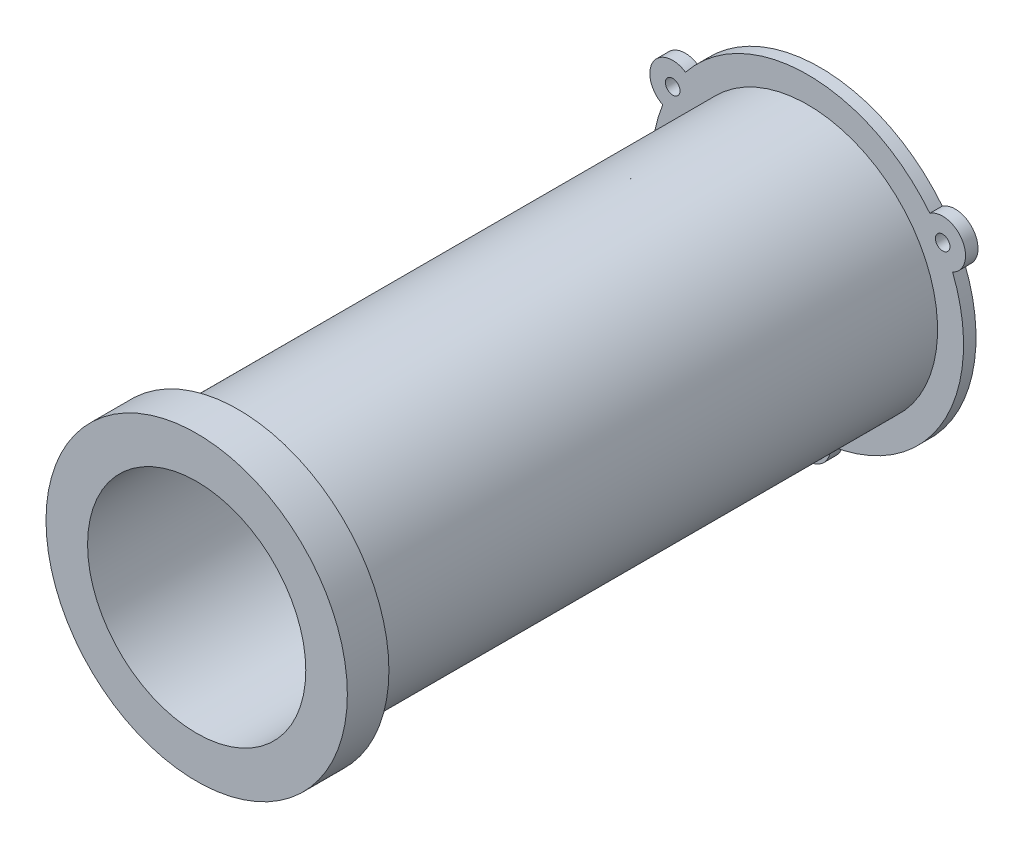
from build123d import *

# Parameters (mm, degrees)
SKETCH_1_R      = 62.5
SKETCH_1_R_2    = 52.5
EXTRUDE_1_DEPTH = 284
SKETCH_2_R      = 72.5
SKETCH_2_R_2    = 52.5
EXTRUDE_2_DEPTH = 10
EXTRUDE_START   = 6
SKETCH_3_R      = 52.5
SKETCH_3_R_2    = 3.5
EXTRUDE_3_DEPTH = 6


with BuildPart() as part:
    # 草图1 → 凸台-拉伸1 (new body)
    with BuildSketch(Plane.XY):
        Circle(SKETCH_1_R)
        Circle(SKETCH_1_R_2, mode=Mode.SUBTRACT)
    extrude(amount=EXTRUDE_1_DEPTH)

    # 草图2 → 凸台-拉伸2 (add, symmetric)
    with BuildSketch(Plane.XY.offset(284)):
        Circle(SKETCH_2_R)
        Circle(SKETCH_2_R_2, mode=Mode.SUBTRACT)
    extrude(amount=EXTRUDE_2_DEPTH, both=True)

    # 草图3 → 凸台-拉伸3 (add)
    with BuildSketch(Plane(origin=(0, 0, 0), x_dir=(-1, 0, 0), z_dir=(0, 0, -1)).offset(EXTRUDE_START)):
        with BuildLine():
            ThreePointArc((10.970382349, -74.193333333), (64.951905284, -37.5), (69.738502633, 27.596036863))
            ThreePointArc((69.738502633, 27.596036863), (74.478184725, 43), (58.768120283, 46.59729647))
            ThreePointArc((58.768120283, 46.59729647), (0, 75), (-58.768120283, 46.59729647))
            ThreePointArc((-58.768120283, 46.59729647), (-74.478184725, 43), (-69.738502633, 27.596036863))
            ThreePointArc((-69.738502633, 27.596036863), (-64.951905284, -37.5), (-10.970382349, -74.193333333))
            ThreePointArc((-10.970382349, -74.193333333), (0, -86), (10.970382349, -74.193333333))
        make_face()
        Circle(SKETCH_3_R, mode=Mode.SUBTRACT)
        with Locations((0, -75)):
            Circle(SKETCH_3_R_2, mode=Mode.SUBTRACT)
        with Locations((-64.951905284, 37.5)):
            Circle(SKETCH_3_R_2, mode=Mode.SUBTRACT)
        with Locations((64.951905284, 37.5)):
            Circle(SKETCH_3_R_2, mode=Mode.SUBTRACT)
    extrude(amount=-EXTRUDE_3_DEPTH)


solid = part.part
